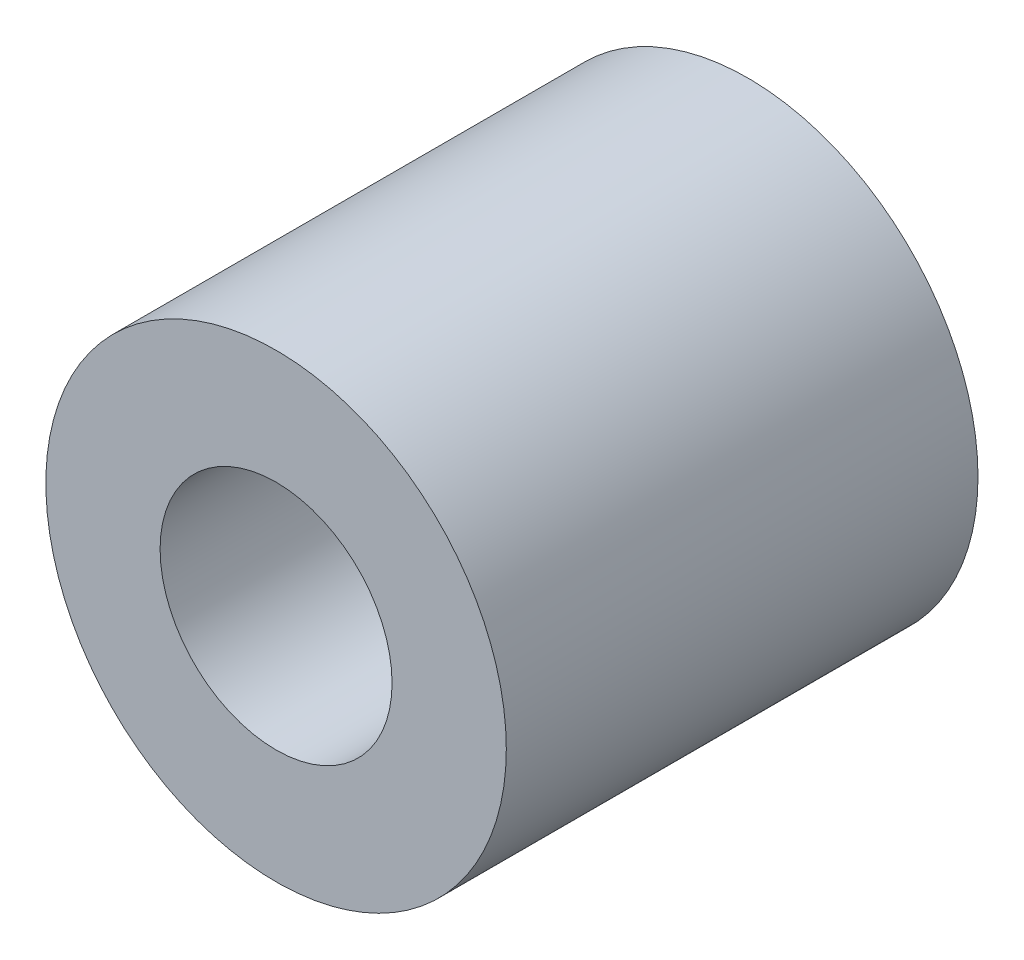
SolidWorks part; units mm, degrees
material "65Mn"
ref_plane "Front Plane" through (0, 0, 0) normal (0, 0, 1) x (1, 0, 0)
ref_plane "Top Plane" through (0, 0, 0) normal (0, 1, 0) x (1, 0, 0)
ref_plane "Right Plane" through (0, 0, 0) normal (1, 0, 0) x (0, 0, -1)
sketch "Sketch1" plane through (0, 0, 0) normal (0, 0, 1) x (1, 0, 0)
  circle A0 centre (0, 0) radius 3
  circle A1 centre (0, 0) radius 5.955
  dimension "D1" = 11.91
  dimension "D2" = 6
extrude "Boss-Extrude1" add sketch "Sketch1" along normal blind 12.2
